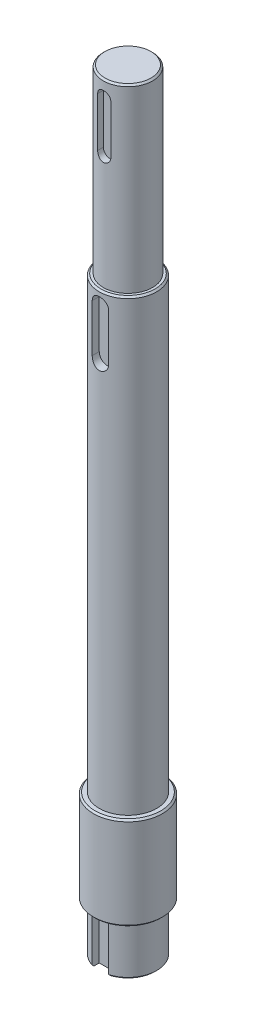
from build123d import *

# Parameters (mm, degrees)
SKETCH1_R           = 17.5
BOSS_EXTRUDE1_DEPTH = 30
SKETCH2_R           = 21
BOSS_EXTRUDE2_DEPTH = 56.5
SKETCH3_R           = 17.5
BOSS_EXTRUDE3_DEPTH = 273.5
SKETCH4_R           = 15
BOSS_EXTRUDE4_DEPTH = 110
CHAMFER1_SIZE       = 1
CHAMFER3_SIZE       = 1
SKETCH5_W           = 10
SKETCH5_H           = 10
CUT_EXTRUDE1_DEPTH  = 30
CUT_EXTRUDE10_DEPTH = 5.5
CUT_EXTRUDE11_DEPTH = 7


with BuildPart() as part:
    # Sketch1 → Boss-Extrude1 (new body)
    with BuildSketch(Plane(origin=(0, 0, 0), x_dir=(1, 0, 0), z_dir=(0, 1, 0))):
        with Locations(Location((0, 0, 0), (0, 0, 270))):
            Circle(SKETCH1_R)
    extrude(amount=BOSS_EXTRUDE1_DEPTH)

    # Sketch2 → Boss-Extrude2 (add)
    with BuildSketch(Plane(origin=(0, 30, 0), x_dir=(1, 0, 0), z_dir=(0, 1, 0))):
        with Locations(Location((0, 0, 0), (0, 0, 270))):
            Circle(SKETCH2_R)
    extrude(amount=BOSS_EXTRUDE2_DEPTH)

    # Sketch3 → Boss-Extrude3 (add)
    with BuildSketch(Plane(origin=(0, 86.5, 0), x_dir=(1, 0, 0), z_dir=(0, 1, 0))):
        with Locations(Location((0, 0, 0), (0, 0, 270))):
            Circle(SKETCH3_R)
    extrude(amount=BOSS_EXTRUDE3_DEPTH)

    # Sketch4 → Boss-Extrude4 (add)
    with BuildSketch(Plane(origin=(0, 360, 0), x_dir=(1, 0, 0), z_dir=(0, 1, 0))):
        with Locations(Location((0, 0, 0), (0, 0, 270))):
            Circle(SKETCH4_R)
    extrude(amount=BOSS_EXTRUDE4_DEPTH)

    # Chamfer1
    chamfer1_edges = [part.edges().sort_by_distance(p)[0] for p in [
        (0, 0, -17.5),
    ]]
    chamfer(chamfer1_edges, length=CHAMFER1_SIZE)

    # Chamfer3
    chamfer3_edges = [part.edges().sort_by_distance(p)[0] for p in [
        (0, 360, -17.5),
        (0, 470, -15),
        (0, 30, -21),
        (0, 86.5, -21),
    ]]
    chamfer(chamfer3_edges, length=CHAMFER3_SIZE)

    # Sketch5 → Cut-Extrude1 (cut)
    with BuildSketch(Plane.XZ):
        with Locations((0, 17.5)):
            Rectangle(SKETCH5_W, SKETCH5_H)
    extrude(amount=-CUT_EXTRUDE1_DEPTH, mode=Mode.SUBTRACT)

    # Sketch8 → Cut-Extrude10 (cut)
    with BuildSketch(Plane.XY.offset(18)):
        with BuildLine():
            Line((5, 351.5), (5, 322.5))
            ThreePointArc((5, 322.5), (0, 317.5), (-5, 322.5))
            Line((-5, 322.5), (-5, 351.5))
            ThreePointArc((-5, 351.5), (0, 356.5), (5, 351.5))
        make_face()
    extrude(amount=-CUT_EXTRUDE10_DEPTH, mode=Mode.SUBTRACT)

    # Sketch9 → Cut-Extrude11 (cut)
    with BuildSketch(Plane.XY.offset(18)):
        with BuildLine():
            Line((4, 460), (4, 430))
            ThreePointArc((4, 430), (0, 426), (-4, 430))
            Line((-4, 430), (-4, 460))
            ThreePointArc((-4, 460), (0, 464), (4, 460))
        make_face()
    extrude(amount=-CUT_EXTRUDE11_DEPTH, mode=Mode.SUBTRACT)


solid = part.part
